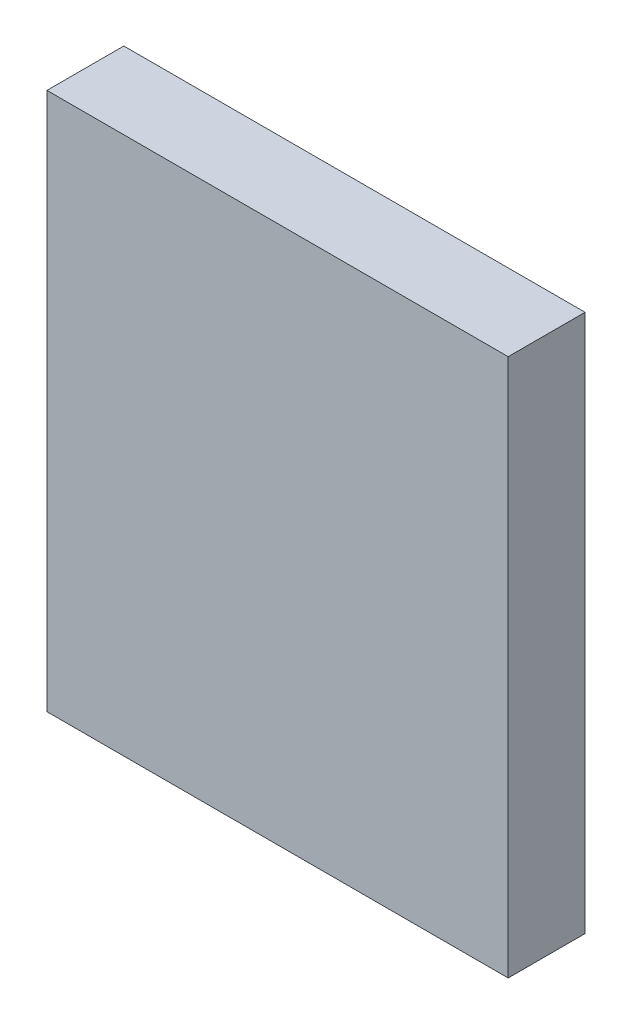
SolidWorks part; units mm, degrees
ref_plane "前视基准面" through (0, 0, 0) normal (0, 0, 1) x (1, 0, 0)
ref_plane "上视基准面" through (0, 0, 0) normal (0, 1, 0) x (1, 0, 0)
ref_plane "右视基准面" through (0, 0, 0) normal (1, 0, 0) x (0, 0, -1)
sketch "草图1" plane through (0, 0, 0) normal (0, 0, 1) x (1, 0, 0)
  line L0 (0, 0) -> (60, 0)
  line L1 (60, 0) -> (60, 70)
  line L2 (60, 70) -> (0, 70)
  line L3 (0, 70) -> (0, 0)
extrude "凸台-拉伸1" add sketch "草图1" along normal blind 10
